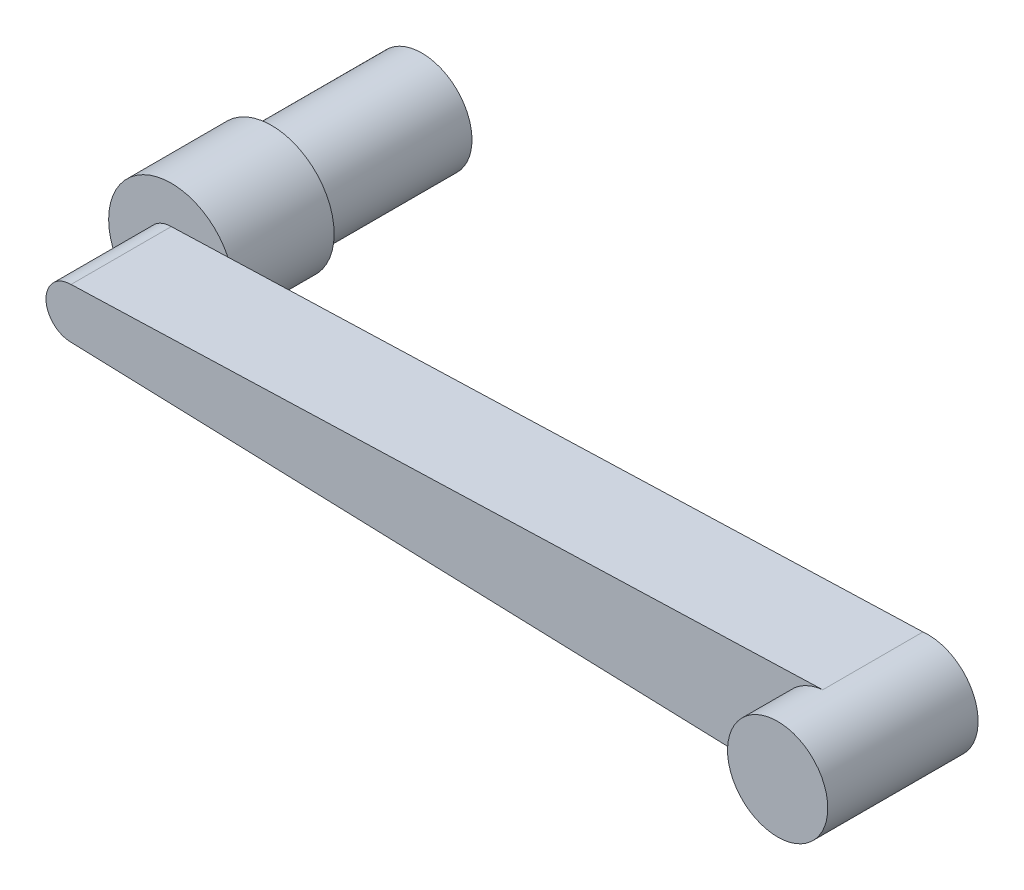
SolidWorks part; units mm, degrees
ref_plane "Front Plane" through (0, 0, 0) normal (0, 0, 1) x (1, 0, 0)
ref_plane "Top Plane" through (0, 0, 0) normal (0, 1, 0) x (1, 0, 0)
ref_plane "Right Plane" through (0, 0, 0) normal (1, 0, 0) x (0, 0, -1)
sketch "Sketch1" plane through (0, 0, 0) normal (0, 0, 1) x (1, 0, 0)
  circle A0 centre (0, 0) radius 1.25
  dimension "D1" = 2.5
extrude "Boss-Extrude1" add sketch "Sketch1" against normal blind 1
sketch "Sketch2" plane through (0, 0, 0) normal (0, 0, 1) x (1, 0, 0)
  circle A0 centre (0, 0) radius 1
  dimension "D1" = 2
extrude "Boss-Extrude2" add sketch "Sketch2" along normal blind 1
sketch "Sketch3" plane through (0, 0, 1) normal (0, 0, 1) x (1, 0, 0)
  line L0 (0, 0.5) -> (15, 0.995)
  line L1 (0, -0.5) -> (15, -0.995)
  arc A0 (0, 0.5) -> (0, -0.5) centre (0, 0) ccw
  arc A2 (15, -0.995) -> (15, 0.995) centre (15.0998, 0) ccw
  dimension "D1" = 1
  dimension "D2" = 15
  dimension "D3" = 2
extrude "Boss-Extrude3" add sketch "Sketch3" along normal blind 2
sketch "Sketch4" plane through (0, 0, 3) normal (0, 0, 1) x (1, 0, 0)
  circle A0 centre (15.0998, 0) radius 1
  dimension "D1" = 2
extrude "Boss-Extrude4" add sketch "Sketch4" along normal blind 1
sketch "Sketch5" plane through (0, 0, 0) normal (0, 0, 1) x (1, 0, 0)
  circle A1 centre (0, 0) radius 1.25
  circle A2 centre (0, 0) radius 1.25
  dimension "D1" = 0
extrude "Boss-Extrude5" add sketch "Sketch5" along normal up to surface (1 mm away) up to face at (-0.1627, 0, 1)
sketch "Sketch6" plane through (0, 0, -1) normal (0, 0, -1) x (-1, 0, 0)
  circle A0 centre (0, 0) radius 1
  dimension "D1" = 2
extrude "Boss-Extrude6" add sketch "Sketch6" along normal blind 3
